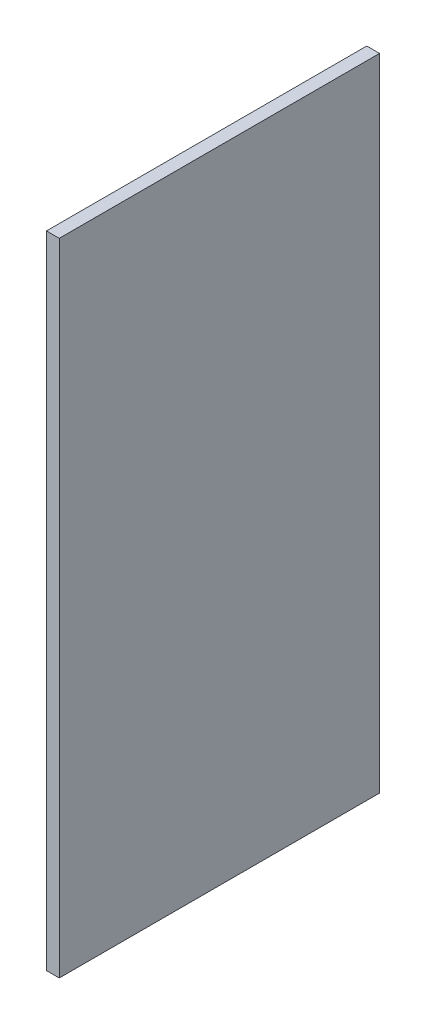
from build123d import *

# Parameters (mm, degrees)
SKETCH_1_W      = 100
SKETCH_1_H      = 200
EXTRUDE_1_DEPTH = 4


with BuildPart() as part:
    # 草图1 → 凸台-拉伸1 (new body)
    with BuildSketch(Plane(origin=(0, 0, 0), x_dir=(0, 0, -1), z_dir=(1, 0, 0))):
        with Locations((50, 100)):
            Rectangle(SKETCH_1_W, SKETCH_1_H)
    extrude(amount=EXTRUDE_1_DEPTH)


solid = part.part
